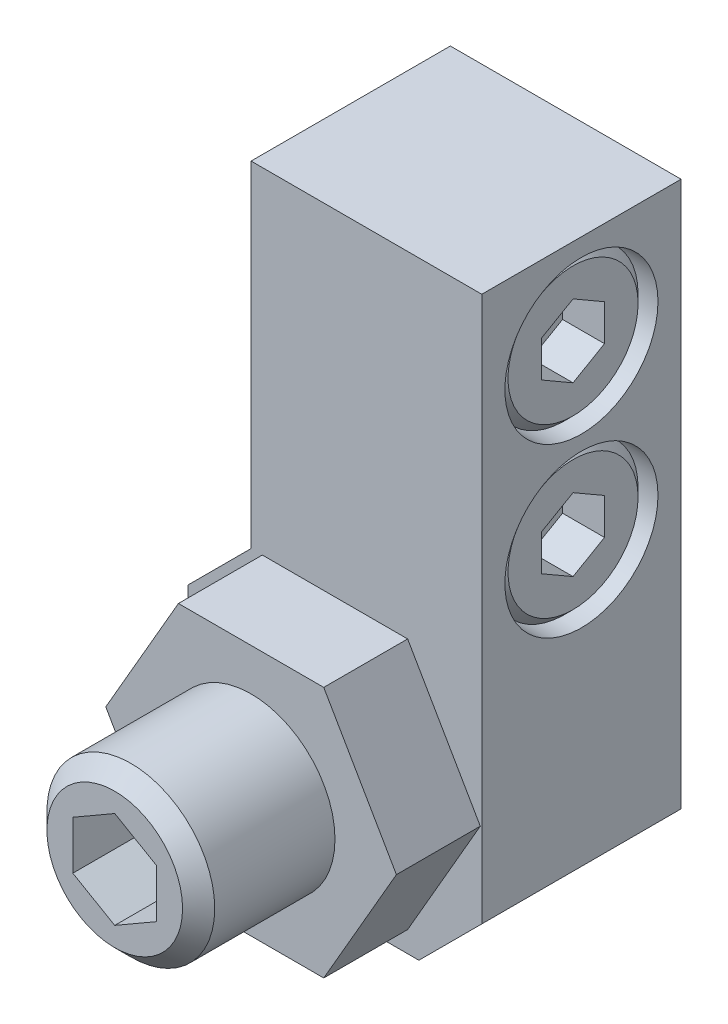
from build123d import *

# Parameters (mm, degrees)
EXTRUDE_1_DEPTH        = 9.5
SKETCH_3_R             = 11
EXTRUDE_2_DEPTH        = 4
SKETCH_4_R             = 11
CUT_EXTRUDE_1_DEPTH    = 4
CUT_EXTRUDE_2_DEPTH    = 4
HOLE_WIZARD_1_D        = 7.3
HOLE_WIZARD_1_DEPTH    = 4.4
PATTERN_LINEAR_1_COUNT = 2
PATTERN_LINEAR_1_PITCH = 8
CUT_EXTRUDE_3_DEPTH    = 2
PATTERN_LINEAR_2_COUNT = 2
PATTERN_LINEAR_2_PITCH = 8


with BuildPart() as part:
    # 草图1 → 凸台-拉伸1 (new body)
    with BuildSketch(Plane.XY):
        Polygon((-14, 3), (-11, 0), (-3, 0), (0, 3), (0, 29), (-11, 29), (-11, 13), (-14, 10), align=None)
    extrude(amount=EXTRUDE_1_DEPTH)

    # 草图3 → 凸台-拉伸2 (add)
    with BuildSketch(Plane.XY.offset(9.5)):
        with Locations(Location((-7, 7, 0), (0, 0, 111.323686263))):
            Circle(SKETCH_3_R)
    extrude(amount=EXTRUDE_2_DEPTH)

    # 草图4 → 切除-拉伸1 (cut)
    with BuildSketch(Plane.XY.offset(9.5)):
        with Locations((-7, 7)):
            Circle(SKETCH_4_R)
        Polygon((-13.9282, 7), (-10.4641, 1.000002798), (-3.5359, 1.000002798), (-0.0718, 7), (-3.5359, 12.999997202), (-10.4641, 12.999997202), align=None, mode=Mode.SUBTRACT)
    extrude(amount=CUT_EXTRUDE_1_DEPTH, mode=Mode.SUBTRACT)

    # 草图2 → 旋转1 (revolve)
    with BuildSketch(Plane(origin=(-7, 0, 0), x_dir=(0, 0, -1), z_dir=(1, 0, 0)), mode=Mode.PRIVATE) as revolve_1_sk:
        Polygon((-20, 7), (-20, 10.233), (-19.233, 11), (1.233, 11), (2, 10.233), (2, 7), align=None)
    revolve(revolve_1_sk.sketch.rotate(Axis((-7, 7, -2), (0, 0, 1)), 270), axis=Axis((-7, 7, -2), (0, 0, 1)))

    # 草图5 → 切除-拉伸2 (cut)
    with BuildSketch(Plane.XY.offset(20)):
        Polygon((-9, 8.154700538), (-9, 5.845299462), (-7, 4.690598923), (-5, 5.845299462), (-5, 8.154700538), (-7, 9.309401077), align=None)
    extrude(amount=-CUT_EXTRUDE_2_DEPTH, mode=Mode.SUBTRACT)

    # 孔1
    with Locations(Plane(origin=(0, 0, 0), x_dir=(0, 0, -1), z_dir=(1, 0, 0))):
        with Locations((-4.75, 24.5)):
            hole_wizard_1 = Hole(HOLE_WIZARD_1_D / 2, depth=HOLE_WIZARD_1_DEPTH)

    # 阵列(线性)1: 孔1 ×2
    with Locations(*[(0, -i * PATTERN_LINEAR_1_PITCH, 0) for i in range(1, PATTERN_LINEAR_1_COUNT)]):
        add(hole_wizard_1, mode=Mode.SUBTRACT)

    # 草图9 → 旋转2 (revolve)
    with BuildSketch(Plane(origin=(0, 24.5, 0), x_dir=(1, 0, 0), z_dir=(0, 1, 0)), mode=Mode.PRIVATE) as revolve_2_sk:
        Polygon((-0.4, -4.75), (-0.4, -7.85), (-0.8, -8.25), (-4.4, -8.25), (-4.4, -4.75), align=None)
    revolve(revolve_2_sk.sketch.rotate(Axis((-4.4, 24.5, 4.75), (1, 0, 0)), 180), axis=Axis((-4.4, 24.5, 4.75), (1, 0, 0)))

    # 草图10 → 旋转3 (revolve)
    with BuildSketch(Plane(origin=(0, 16.5, 0), x_dir=(1, 0, 0), z_dir=(0, 1, 0)), mode=Mode.PRIVATE) as revolve_3_sk:
        Polygon((-0.4, -4.75), (-0.4, -7.85), (-0.8, -8.25), (-4.4, -8.25), (-4.4, -4.75), align=None)
    revolve(revolve_3_sk.sketch.rotate(Axis((-4.4, 16.5, 4.75), (1, 0, 0)), 180), axis=Axis((-4.4, 16.5, 4.75), (1, 0, 0)))

    # 草图11 → 切除-拉伸3 (cut)
    with BuildSketch(Plane(origin=(-0.4, 0, 0), x_dir=(0, 0, -1), z_dir=(1, 0, 0))):
        Polygon((-6.25, 25.366025404), (-6.25, 23.633974596), (-4.75, 22.767949192), (-3.25, 23.633974596), (-3.25, 25.366025404), (-4.75, 26.232050808), align=None)
    cut_extrude_3 = extrude(amount=-CUT_EXTRUDE_3_DEPTH, mode=Mode.SUBTRACT)

    # 阵列(线性)2: 切除-拉伸3 ×2
    with Locations(*[(0, -i * PATTERN_LINEAR_2_PITCH, 0) for i in range(1, PATTERN_LINEAR_2_COUNT)]):
        add(cut_extrude_3, mode=Mode.SUBTRACT)


solid = part.part
